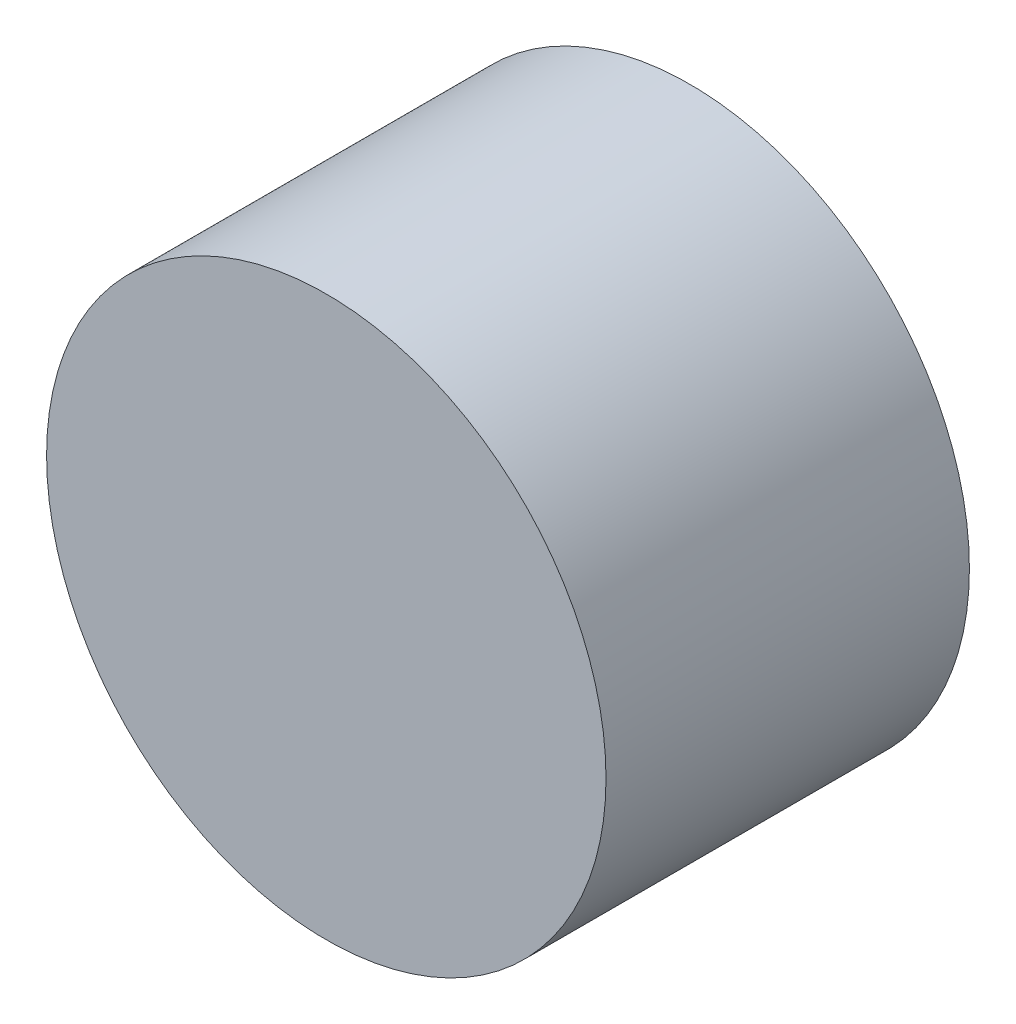
from build123d import *

# Parameters (mm, degrees)
SKETCH1_R           = 7.6973628
BOSS_EXTRUDE1_DEPTH = 10


with BuildPart() as part:
    # Sketch1 → Boss-Extrude1 (new body)
    with BuildSketch(Plane.XY):
        with Locations((-17.055797946, 0)):
            Circle(SKETCH1_R)
    extrude(amount=BOSS_EXTRUDE1_DEPTH)


solid = part.part
